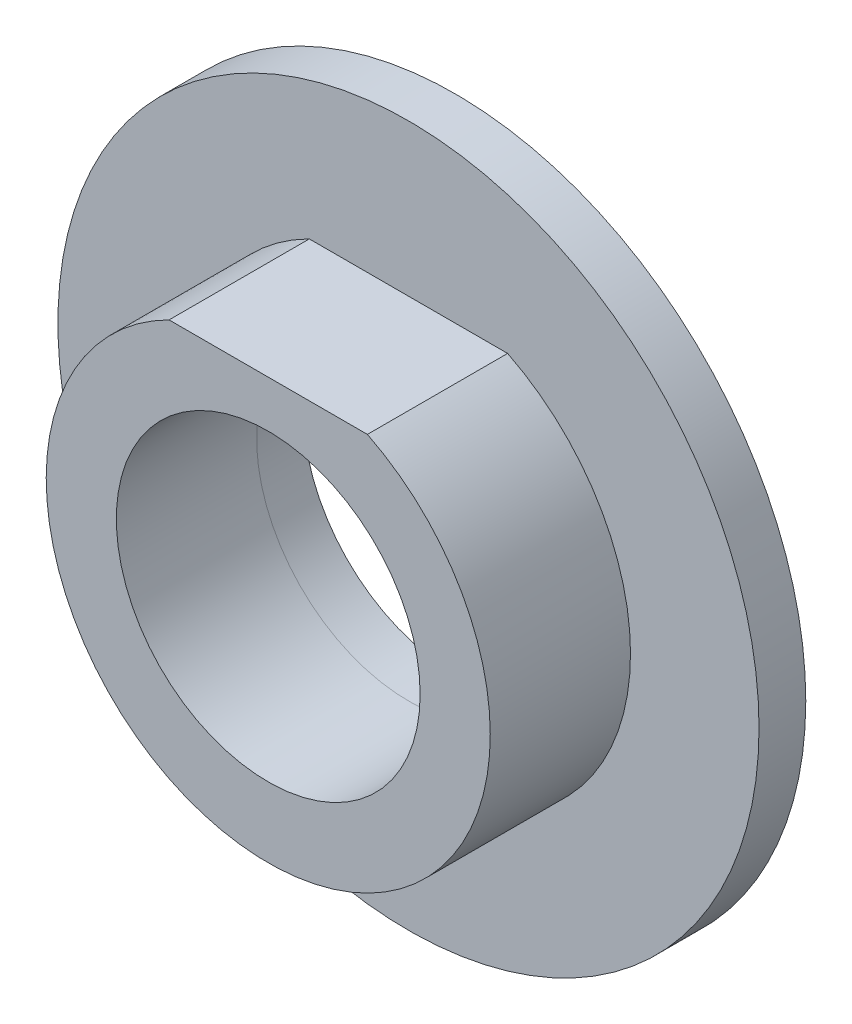
from build123d import *

# Parameters (mm, degrees)
SKETCH_1_R          = 15
EXTRUDE_1_DEPTH     = 2
SKETCH_2_R          = 9.5
EXTRUDE_2_DEPTH     = 6
SKETCH_3_R          = 6.5
CUT_EXTRUDE_1_DEPTH = 15
CUT_EXTRUDE_2_DEPTH = 6


with BuildPart() as part:
    # 草图1 → 凸台-拉伸1 (new body)
    with BuildSketch(Plane.XY):
        Circle(SKETCH_1_R)
    extrude(amount=EXTRUDE_1_DEPTH)


with BuildPart() as body_2:
    # 草图2 → 凸台-拉伸2 (new body)
    with BuildSketch(Plane.XY.offset(2)):
        Circle(SKETCH_2_R)
    extrude(amount=EXTRUDE_2_DEPTH)


with BuildPart() as cut_extrude_1_tool:
    # 草图3 → 切除-拉伸1 (new body)
    with BuildSketch(Plane.XY.offset(8)):
        Circle(SKETCH_3_R)
    extrude(amount=-CUT_EXTRUDE_1_DEPTH)


with BuildPart() as part_1:
    add(part.part)

    # 切除-拉伸1: cut by cut_extrude_1_tool
    add(cut_extrude_1_tool.part, mode=Mode.SUBTRACT)


with BuildPart() as body_2_1:
    add(body_2.part)

    # 切除-拉伸1: cut by cut_extrude_1_tool
    add(cut_extrude_1_tool.part, mode=Mode.SUBTRACT)

    # 草图4 → 切除-拉伸2 (cut)
    with BuildSketch(Plane.XY.offset(8)):
        with BuildLine():
            Line((-4.242640687, 8.5), (4.242640687, 8.5))
            ThreePointArc((4.242640687, 8.5), (0, 9.5), (-4.242640687, 8.5))
        make_face()
    extrude(amount=-CUT_EXTRUDE_2_DEPTH, mode=Mode.SUBTRACT)


solid = Compound([part_1.part, body_2_1.part])
